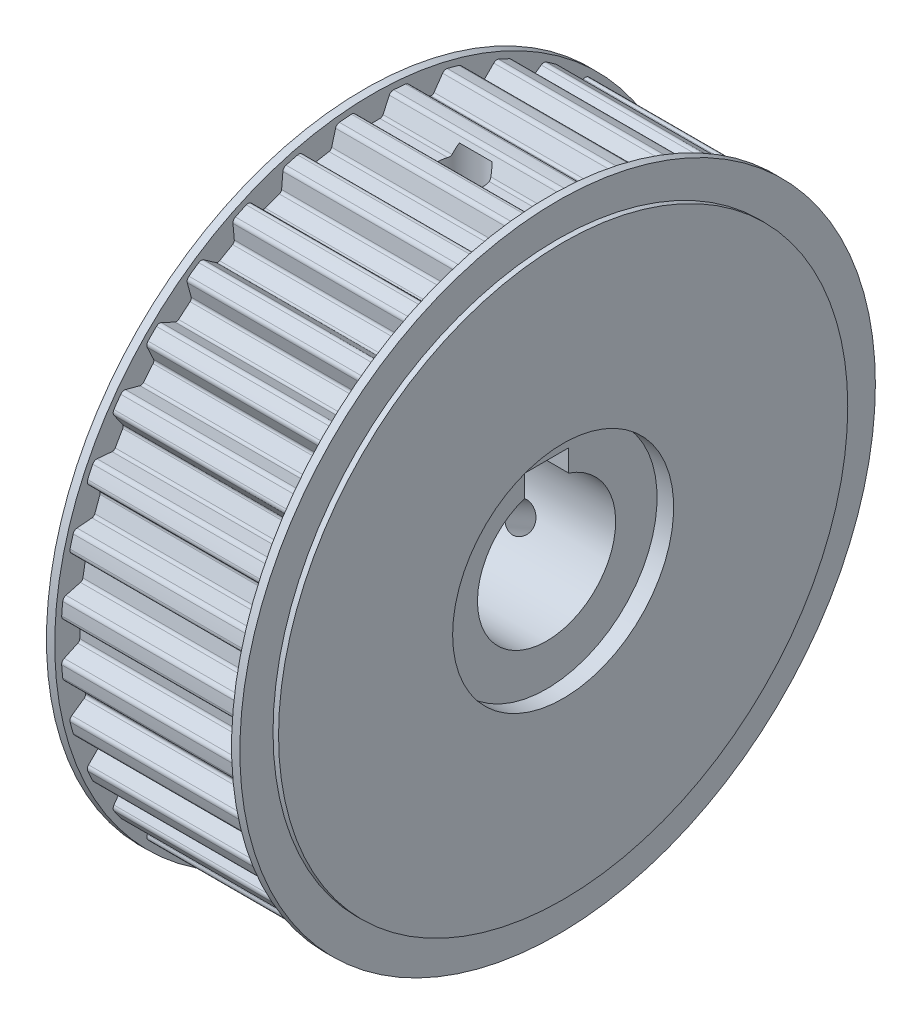
from build123d import *

# Parameters (mm, degrees)
SKETCH_1_R                       = 56.37
EXTRUDE_1_DEPTH                  = 16
CUT_EXTRUDE_2_DEPTH              = 32
FILLET_1_R                       = 0.6
FILLET_2_R                       = 0.8
PATTERN_CIRCULAR_1_COUNT         = 36
FILLET_1_OF_PATTERN_CIRCULAR_1_R = 0.6
FILLET_2_OF_PATTERN_CIRCULAR_1_R = 0.8
SKETCH_6_R                       = 57.5
EXTRUDE_2_DEPTH                  = 1.5
SKETCH_7_R                       = 51.5
EXTRUDE_3_DEPTH                  = 1
SKETCH_8_R                       = 12.5
CUT_EXTRUDE_1_DEPTH              = 90.339241098
SKETCH_11_R                      = 20
CUT_EXTRUDE_3_DEPTH              = 3
SKETCH_12_W                      = 8
SKETCH_12_H                      = 5.692858801
CUT_EXTRUDE_4_DEPTH              = 90.339241098
SKETCH_15_R                      = 4
CUT_EXTRUDE_5_DEPTH              = 30
PATTERN_CIRCULAR_2_COUNT         = 2
PATTERN_CIRCULAR_2_ANGLE         = 120


with BuildPart() as part:
    # 草图1 → 拉伸1 (new, symmetric)
    with BuildSketch(Plane(origin=(0, 0, 0), x_dir=(0, 0, -1), z_dir=(1, 0, 0))):
        Circle(SKETCH_1_R)
    extrude(amount=EXTRUDE_1_DEPTH, both=True)

    # 草图2 → Cut-Extrude 2 (cut)
    with BuildSketch(Plane(origin=(16, 0, 0), x_dir=(0, 0, -1), z_dir=(1, 0, 0))):
        with BuildLine():
            Line((-3.285, 56.274200794), (-1.744225866, 52.97))
            Line((-1.744225866, 52.97), (1.744225866, 52.97))
            Line((1.744225866, 52.97), (3.285, 56.274200794))
            ThreePointArc((3.285, 56.274200794), (0, 56.37), (-3.285, 56.274200794))
        make_face()
    cut_extrude_2 = extrude(amount=-CUT_EXTRUDE_2_DEPTH, mode=Mode.SUBTRACT)

    # 圆角1
    fillet_1_edges = [part.edges().sort_by_distance(p)[0] for p in [
        (0, 52.97, 1.744225866),
        (0, 52.97, -1.744225866),
    ]]
    fillet(fillet_1_edges, radius=FILLET_1_R)

    # 圆角2
    fillet_2_edges = [part.edges().sort_by_distance(p)[0] for p in [
        (0, 56.274200794, 3.285),
        (0, 56.274200794, -3.285),
    ]]
    fillet(fillet_2_edges, radius=FILLET_2_R)

    # 阵列(圆周)1: Cut-Extrude 2 ×36 about axis
    pattern_circular_1_axis = Axis((0, 0, 0), (1, 0, 0))
    for i in range(1, PATTERN_CIRCULAR_1_COUNT):
        add(cut_extrude_2.rotate(pattern_circular_1_axis, i * 360 / PATTERN_CIRCULAR_1_COUNT), mode=Mode.SUBTRACT)

    # 圆角1 of 阵列(圆周)1
    fillet_1_of_pattern_circular_1_edges = [part.edges().sort_by_distance(p)[0] for p in [
        (0, 51.862385034, 10.915871127),
        (0, 52.46814832, 7.480416815),
        (0, 49.178957742, 19.755843167),
        (0, 50.372078504, 16.477770817),
        (0, 45.001252706, 27.99554391),
        (0, 46.745478571, 24.97445609),
        (0, 39.456207377, 35.384614217),
        (0, 41.698540927, 32.712305153),
        (0, 32.712305153, 41.698540927),
        (0, 35.384614217, 39.456207377),
        (0, 24.97445609, 46.745478571),
        (0, 27.99554391, 45.001252706),
        (0, 16.477770817, 50.372078504),
        (0, 19.755843167, 49.178957742),
        (0, 7.480416815, 52.46814832),
        (0, 10.915871127, 51.862385034),
        (0, -1.744225866, 52.97),
        (0, 1.744225866, 52.97),
        (0, -10.915871127, 51.862385034),
        (0, -7.480416815, 52.46814832),
        (0, -19.755843167, 49.178957742),
        (0, -16.477770817, 50.372078504),
        (0, -27.99554391, 45.001252706),
        (0, -24.97445609, 46.745478571),
        (0, -35.384614217, 39.456207377),
        (0, -32.712305153, 41.698540927),
        (0, -41.698540927, 32.712305153),
        (0, -39.456207377, 35.384614217),
        (0, -46.745478571, 24.97445609),
        (0, -45.001252706, 27.99554391),
        (0, -50.372078504, 16.477770817),
        (0, -49.178957742, 19.755843167),
        (0, -52.46814832, 7.480416815),
        (0, -51.862385034, 10.915871127),
        (0, -52.97, -1.744225866),
        (0, -52.97, 1.744225866),
        (0, -51.862385034, -10.915871127),
        (0, -52.46814832, -7.480416815),
        (0, -49.178957742, -19.755843167),
        (0, -50.372078504, -16.477770817),
        (0, -45.001252706, -27.99554391),
        (0, -46.745478571, -24.97445609),
        (0, -39.456207377, -35.384614217),
        (0, -41.698540927, -32.712305153),
        (0, -32.712305153, -41.698540927),
        (0, -35.384614217, -39.456207377),
        (0, -24.97445609, -46.745478571),
        (0, -27.99554391, -45.001252706),
        (0, -16.477770817, -50.372078504),
        (0, -19.755843167, -49.178957742),
        (0, -7.480416815, -52.46814832),
        (0, -10.915871127, -51.862385034),
        (0, 1.744225866, -52.97),
        (0, -1.744225866, -52.97),
        (0, 10.915871127, -51.862385034),
        (0, 7.480416815, -52.46814832),
        (0, 19.755843167, -49.178957742),
        (0, 16.477770817, -50.372078504),
        (0, 27.99554391, -45.001252706),
        (0, 24.97445609, -46.745478571),
        (0, 35.384614217, -39.456207377),
        (0, 32.712305153, -41.698540927),
        (0, 41.698540927, -32.712305153),
        (0, 39.456207377, -35.384614217),
        (0, 46.745478571, -24.97445609),
        (0, 45.001252706, -27.99554391),
        (0, 50.372078504, -16.477770817),
        (0, 49.178957742, -19.755843167),
        (0, 52.46814832, -7.480416815),
        (0, 51.862385034, -10.915871127),
    ]]
    fillet(fillet_1_of_pattern_circular_1_edges, radius=FILLET_1_OF_PATTERN_CIRCULAR_1_R)

    # 圆角2 of 阵列(圆周)1
    fillet_2_of_pattern_circular_1_edges = [part.edges().sort_by_distance(p)[0] for p in [
        (0, 54.848834973, 13.007005886),
        (0, 55.9897035, 6.536818949),
        (0, 51.756915056, 22.33380048),
        (0, 54.003987398, 16.160019962),
        (0, 47.092387465, 30.981993848),
        (0, 50.377387465, 25.292206946),
        (0, 40.996981511, 38.688815011),
        (0, 45.220096107, 33.65590302),
        (0, 33.65590302, 45.220096107),
        (0, 38.688815011, 40.996981511),
        (0, 25.292206946, 50.377387465),
        (0, 30.981993848, 47.092387465),
        (0, 16.160019962, 54.003987398),
        (0, 22.33380048, 51.756915056),
        (0, 6.536818949, 55.9897035),
        (0, 13.007005886, 54.848834973),
        (0, -3.285, 56.274200794),
        (0, 3.285, 56.274200794),
        (0, -13.007005886, 54.848834973),
        (0, -6.536818949, 55.9897035),
        (0, -22.33380048, 51.756915056),
        (0, -16.160019962, 54.003987398),
        (0, -30.981993848, 47.092387465),
        (0, -25.292206946, 50.377387465),
        (0, -38.688815011, 40.996981511),
        (0, -33.65590302, 45.220096107),
        (0, -45.220096107, 33.65590302),
        (0, -40.996981511, 38.688815011),
        (0, -50.377387465, 25.292206946),
        (0, -47.092387465, 30.981993848),
        (0, -54.003987398, 16.160019962),
        (0, -51.756915056, 22.33380048),
        (0, -55.9897035, 6.536818949),
        (0, -54.848834973, 13.007005886),
        (0, -56.274200794, -3.285),
        (0, -56.274200794, 3.285),
        (0, -54.848834973, -13.007005886),
        (0, -55.9897035, -6.536818949),
        (0, -51.756915056, -22.33380048),
        (0, -54.003987398, -16.160019962),
        (0, -47.092387465, -30.981993848),
        (0, -50.377387465, -25.292206946),
        (0, -40.996981511, -38.688815011),
        (0, -45.220096107, -33.65590302),
        (0, -33.65590302, -45.220096107),
        (0, -38.688815011, -40.996981511),
        (0, -25.292206946, -50.377387465),
        (0, -30.981993848, -47.092387465),
        (0, -16.160019962, -54.003987398),
        (0, -22.33380048, -51.756915056),
        (0, -6.536818949, -55.9897035),
        (0, -13.007005886, -54.848834973),
        (0, 3.285, -56.274200794),
        (0, -3.285, -56.274200794),
        (0, 13.007005886, -54.848834973),
        (0, 6.536818949, -55.9897035),
        (0, 22.33380048, -51.756915056),
        (0, 16.160019962, -54.003987398),
        (0, 30.981993848, -47.092387465),
        (0, 25.292206946, -50.377387465),
        (0, 38.688815011, -40.996981511),
        (0, 33.65590302, -45.220096107),
        (0, 45.220096107, -33.65590302),
        (0, 40.996981511, -38.688815011),
        (0, 50.377387465, -25.292206946),
        (0, 47.092387465, -30.981993848),
        (0, 54.003987398, -16.160019962),
        (0, 51.756915056, -22.33380048),
        (0, 55.9897035, -6.536818949),
        (0, 54.848834973, -13.007005886),
    ]]
    fillet(fillet_2_of_pattern_circular_1_edges, radius=FILLET_2_OF_PATTERN_CIRCULAR_1_R)

    # 草图6 → 凸台-拉伸2 (add)
    with BuildSketch(Plane(origin=(16, 0, 0), x_dir=(0, 0, -1), z_dir=(1, 0, 0))):
        Circle(SKETCH_6_R)
    extrude_2 = extrude(amount=EXTRUDE_2_DEPTH)

    # 草图7 → 凸台-拉伸3 (add)
    with BuildSketch(Plane(origin=(17.5, 0, 0), x_dir=(0, 0, -1), z_dir=(1, 0, 0))):
        Circle(SKETCH_7_R)
    extrude_3 = extrude(amount=EXTRUDE_3_DEPTH)

    # 镜向2: 凸台-拉伸2, 凸台-拉伸3 across plane
    add(extrude_2.mirror(Plane(origin=(0, 0, 0), x_dir=(0, 0, 1), z_dir=(1, 0, 0))))
    add(extrude_3.mirror(Plane(origin=(0, 0, 0), x_dir=(0, 0, 1), z_dir=(1, 0, 0))))

    # 草图8 → 切除-拉伸1 (cut, through all)
    with BuildSketch(Plane.ZY.offset(18.5)):
        Circle(SKETCH_8_R)
    extrude(amount=-CUT_EXTRUDE_1_DEPTH, mode=Mode.SUBTRACT)

    # 草图11 → 切除-拉伸3 (cut)
    with BuildSketch(Plane.ZY.offset(18.5)):
        Circle(SKETCH_11_R)
    cut_extrude_3 = extrude(amount=-CUT_EXTRUDE_3_DEPTH, mode=Mode.SUBTRACT)

    # 镜向3: 切除-拉伸3 across plane
    add(cut_extrude_3.mirror(Plane(origin=(0, 0, 0), x_dir=(0, 0, 1), z_dir=(1, 0, 0))), mode=Mode.SUBTRACT)

    # 草图12 → 切除-拉伸4 (cut, through all)
    with BuildSketch(Plane.ZY.offset(18.5)):
        with Locations((0, 12.9535706)):
            Rectangle(SKETCH_12_W, SKETCH_12_H)
    extrude(amount=-CUT_EXTRUDE_4_DEPTH, mode=Mode.SUBTRACT)

    # 草图13 → M6 螺纹孔1 (revolve, cut)
    with BuildSketch(Plane(origin=(0, 55, 0), x_dir=(0, 0, 1), z_dir=(1, 0, 0))):
        Polygon((0, 0), (0, 51.502151548), (2.5, 50), (2.5, 0), align=None)
    hole_wizard_m6_1 = revolve(axis=Axis((0, 61.35, 0), (0, -1, 0)), mode=Mode.SUBTRACT)

    # 草图15 → 切除-拉伸5 (cut)
    with BuildSketch(Plane(origin=(0, 55, 0), x_dir=(1, 0, 0), z_dir=(0, 1, 0))):
        with Locations(Location((0, 0, 0), (0, 0, 270))):
            Circle(SKETCH_15_R)
    cut_extrude_5 = extrude(amount=-CUT_EXTRUDE_5_DEPTH, mode=Mode.SUBTRACT)

    # 阵列(圆周)2: M6 螺纹孔1, 切除-拉伸5 ×2 about axis
    pattern_circular_2_axis = Axis((18.5, 0, 0), (-1, 0, 0))
    add([hole_wizard_m6_1.rotate(pattern_circular_2_axis, i * PATTERN_CIRCULAR_2_ANGLE / (PATTERN_CIRCULAR_2_COUNT - 1)) for i in range(1, PATTERN_CIRCULAR_2_COUNT)], mode=Mode.SUBTRACT)
    add([cut_extrude_5.rotate(pattern_circular_2_axis, i * PATTERN_CIRCULAR_2_ANGLE / (PATTERN_CIRCULAR_2_COUNT - 1)) for i in range(1, PATTERN_CIRCULAR_2_COUNT)], mode=Mode.SUBTRACT)


solid = part.part
